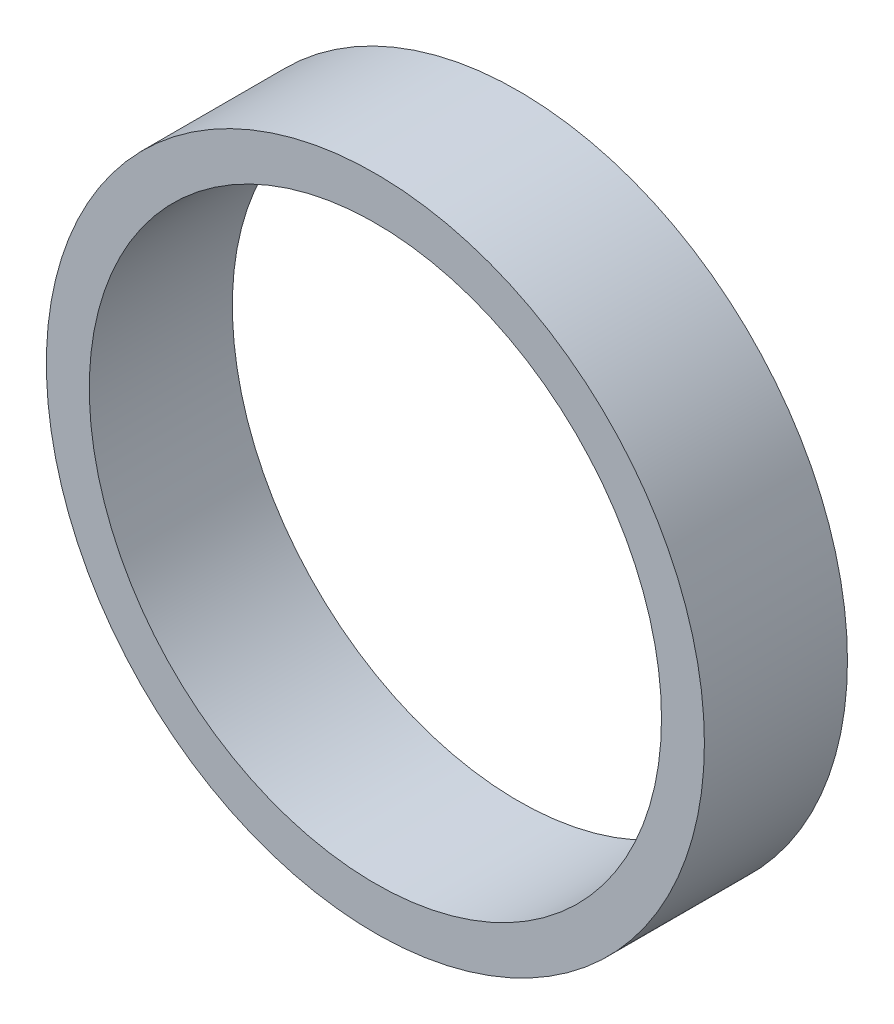
from build123d import *

# Parameters (mm, degrees)
SKETCH1_R           = 115
SKETCH1_R_2         = 100
BOSS_EXTRUDE1_DEPTH = 25


with BuildPart() as part:
    # Sketch1 → Boss-Extrude1 (new, symmetric)
    with BuildSketch(Plane.XY):
        Circle(SKETCH1_R)
        Circle(SKETCH1_R_2, mode=Mode.SUBTRACT)
    extrude(amount=BOSS_EXTRUDE1_DEPTH, both=True)


solid = part.part
